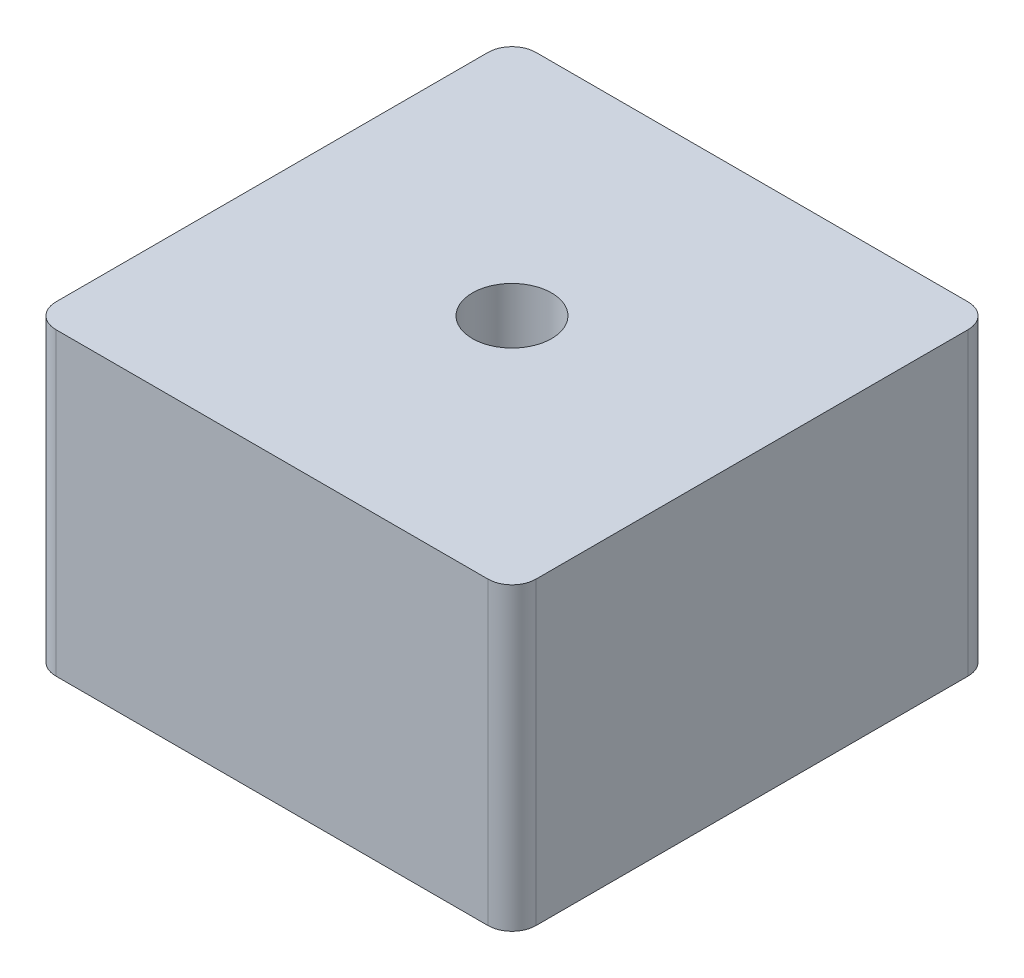
from build123d import *

# Parameters (mm, degrees)
SKETCH1_W           = 20
SKETCH1_H           = 20
BOSS_EXTRUDE1_DEPTH = 12.5
M4_TAPPED_HOLE1_D   = 3.3
FILLET1_R           = 1


with BuildPart() as part:
    # Sketch1 → Boss-Extrude1 (new body)
    with BuildSketch(Plane(origin=(0, 0, 0), x_dir=(1, 0, 0), z_dir=(0, 1, 0))):
        Rectangle(SKETCH1_W, SKETCH1_H)
    extrude(amount=BOSS_EXTRUDE1_DEPTH)

    # M4 Tapped Hole1 (through all)
    with Locations(Plane(origin=(0, 12.5, 0), x_dir=(1, 0, 0), z_dir=(0, 1, 0))):
        with Locations((0, 0)):
            Hole(M4_TAPPED_HOLE1_D / 2)

    # Fillet1
    fillet1_edges = [part.edges().sort_by_distance(p)[0] for p in [
        (10, 6.25, 10),
        (-10, 6.25, 10),
        (-10, 6.25, -10),
        (10, 6.25, -10),
    ]]
    fillet(fillet1_edges, radius=FILLET1_R)


solid = part.part
